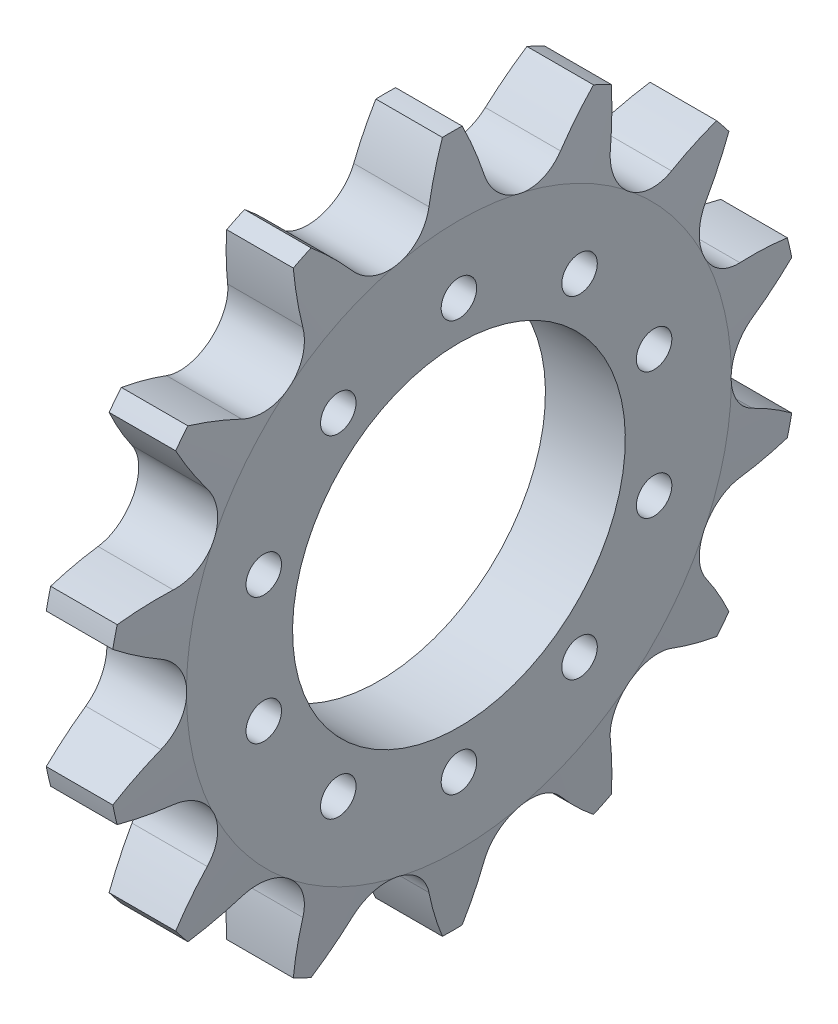
SolidWorks part; units mm, degrees
material "铸造合金钢"
ref_plane "Front Plane" through (0, 0, 0) normal (0, 0, 1) x (1, 0, 0)
ref_plane "Top Plane" through (0, 0, 0) normal (0, 1, 0) x (1, 0, 0)
ref_plane "Right Plane" through (0, 0, 0) normal (1, 0, 0) x (0, 0, -1)
sketch "Sketch1" plane through (0, 0, 0) normal (0, 0, 1) x (1, 0, 0)
  line L0 (15, 156) -> (-15, 156)
  line L1 (0, -55) -> (0, 55) construction
  line L2 (-15, 156) -> (-18, 122.845)
  line L3 (-18, 122.845) -> (-18, 75)
  line L4 (-18, 75) -> (18, 75)
  line L5 (0, 55.746) -> (0, 0) construction
  line L6 (0, 0) -> (-42.4498, 0) construction
  line L7 (18, 122.845) -> (18, 75)
  line L8 (15, 156) -> (18, 122.845)
  line L9 (15, -156) -> (18, -122.845) construction
  line L10 (18, -122.845) -> (18, -75) construction
  line L11 (-18, -75) -> (18, -75) construction
  line L12 (-18, -122.845) -> (-18, -75) construction
  line L13 (-15, -156) -> (-18, -122.845) construction
  line L14 (15, -156) -> (-15, -156) construction
  point P12 (0, 75)
  point P14 (0, 156)
  point P20 (0, -156)
  point P21 (0, -75)
  dimension "D1" = 30
  dimension "D2" = 36
  dimension "D3" = 312
  dimension "D4" = 245.69
  dimension "D5" = 150
revolve "Revolve1" add sketch "Sketch1" angle 360 about L6
sketch "Sketch3" plane through (0, 0, 0) normal (1, 0, 0) x (0, 0, -1)
  line L1 (-159.75, 0) -> (159.75, 0) construction
  line L2 (0, 159.75) -> (0, -159.75) construction
  circle A0 centre (0, 0) radius 196.1047
  arc A3 (153.6801, 30.8707) -> (151.8553, 38.8657) centre (0, 0) ccw
  arc A4 (125.0666, 94.4928) -> (119.9537, 100.9043) centre (0, 0) ccw
  arc A5 (71.6822, 139.3995) -> (64.2938, 142.9576) centre (0, 0) ccw
  arc A6 (4.1003, 156.6964) -> (-4.1003, 156.6964) centre (0, 0) ccw
  arc A7 (-64.2938, 142.9576) -> (-71.6822, 139.3995) centre (0, 0) ccw
  arc A8 (-119.9537, 100.9043) -> (-125.0666, 94.4928) centre (0, 0) ccw
  arc A9 (-151.8553, 38.8657) -> (-153.6801, 30.8707) centre (0, 0) ccw
  arc A10 (-153.6801, -30.8707) -> (-151.8553, -38.8657) centre (0, 0) ccw
  arc A11 (-125.0666, -94.4928) -> (-119.9537, -100.9043) centre (0, 0) ccw
  arc A12 (-71.6822, -139.3995) -> (-64.2938, -142.9576) centre (0, 0) ccw
  arc A13 (-4.1003, -156.6964) -> (4.1003, -156.6964) centre (0, 0) ccw
  arc A14 (64.2938, -142.9576) -> (71.6822, -139.3995) centre (0, 0) ccw
  arc A15 (119.9537, -100.9043) -> (125.0666, -94.4928) centre (0, 0) ccw
  arc A16 (151.8553, -38.8657) -> (153.6801, -30.8707) centre (0, 0) ccw
  arc A17 (153.6801, -30.8707) -> (133.2631, -17.6303) centre (65.3353, -144.7381) ccw
  arc A18 (133.2631, 17.6303) -> (133.2631, -17.6303) centre (142.685, 0) ccw
  arc A19 (133.2631, 17.6303) -> (153.6801, 30.8707) centre (65.3353, 144.7381) ccw
  arc A20 (151.8553, 38.8657) -> (127.7155, 41.9363) centre (121.6646, -102.0566) ccw
  arc A21 (112.4164, 73.7051) -> (127.7155, 41.9363) centre (128.5547, 61.9087) ccw
  arc A22 (112.4164, 73.7051) -> (125.0666, 94.4928) centre (-3.9344, 158.7524) ccw
  arc A23 (119.9537, 100.9043) -> (96.8722, 93.197) centre (153.8967, -39.1615) ccw
  arc A24 (69.3043, 115.1817) -> (96.8722, 93.197) centre (88.9626, 111.5556) ccw
  arc A25 (69.3043, 115.1817) -> (71.6822, 139.3995) centre (-72.4249, 141.3239) ccw
  arc A26 (64.2938, 142.9576) -> (46.8421, 125.9988) centre (155.6477, 31.49) ccw
  arc A27 (12.4655, 133.8451) -> (46.8421, 125.9988) centre (31.7504, 139.1076) ccw
  arc A28 (12.4655, 133.8451) -> (4.1003, 156.6964) centre (-126.5707, 95.9045) ccw
  arc A29 (-4.1003, 156.6964) -> (-12.4655, 133.8451) centre (126.5707, 95.9045) ccw
  arc A30 (-46.8421, 125.9988) -> (-12.4655, 133.8451) centre (-31.7504, 139.1076) ccw
  arc A31 (-46.8421, 125.9988) -> (-64.2938, 142.9576) centre (-155.6477, 31.49) ccw
  arc A32 (-71.6822, 139.3995) -> (-69.3043, 115.1817) centre (72.4249, 141.3239) ccw
  arc A33 (-96.8722, 93.197) -> (-69.3043, 115.1817) centre (-88.9626, 111.5556) ccw
  arc A34 (-96.8722, 93.197) -> (-119.9537, 100.9043) centre (-153.8967, -39.1615) ccw
  arc A35 (-125.0666, 94.4928) -> (-112.4164, 73.7051) centre (3.9344, 158.7524) ccw
  arc A36 (-127.7155, 41.9363) -> (-112.4164, 73.7051) centre (-128.5547, 61.9087) ccw
  arc A37 (-127.7155, 41.9363) -> (-151.8553, 38.8657) centre (-121.6646, -102.0566) ccw
  arc A38 (-153.6801, 30.8707) -> (-133.2631, 17.6303) centre (-65.3353, 144.7381) ccw
  arc A39 (-133.2631, -17.6303) -> (-133.2631, 17.6303) centre (-142.685, 0) ccw
  arc A40 (-133.2631, -17.6303) -> (-153.6801, -30.8707) centre (-65.3353, -144.7381) ccw
  arc A41 (-151.8553, -38.8657) -> (-127.7155, -41.9363) centre (-121.6646, 102.0566) ccw
  arc A42 (-112.4164, -73.7051) -> (-127.7155, -41.9363) centre (-128.5547, -61.9087) ccw
  arc A43 (-112.4164, -73.7051) -> (-125.0666, -94.4928) centre (3.9344, -158.7524) ccw
  arc A44 (-119.9537, -100.9043) -> (-96.8722, -93.197) centre (-153.8967, 39.1615) ccw
  arc A45 (-69.3043, -115.1817) -> (-96.8722, -93.197) centre (-88.9626, -111.5556) ccw
  arc A46 (-69.3043, -115.1817) -> (-71.6822, -139.3995) centre (72.4249, -141.3239) ccw
  arc A47 (-64.2938, -142.9576) -> (-46.8421, -125.9988) centre (-155.6477, -31.49) ccw
  arc A48 (-12.4655, -133.8451) -> (-46.8421, -125.9988) centre (-31.7504, -139.1076) ccw
  arc A49 (-12.4655, -133.8451) -> (-4.1003, -156.6964) centre (126.5707, -95.9045) ccw
  arc A50 (4.1003, -156.6964) -> (12.4655, -133.8451) centre (-126.5707, -95.9045) ccw
  arc A51 (46.8421, -125.9988) -> (12.4655, -133.8451) centre (31.7504, -139.1076) ccw
  arc A52 (46.8421, -125.9988) -> (64.2938, -142.9576) centre (155.6477, -31.49) ccw
  arc A53 (71.6822, -139.3995) -> (69.3043, -115.1817) centre (-72.4249, -141.3239) ccw
  arc A54 (96.8722, -93.197) -> (69.3043, -115.1817) centre (88.9626, -111.5556) ccw
  arc A55 (96.8722, -93.197) -> (119.9537, -100.9043) centre (153.8967, 39.1615) ccw
  arc A56 (125.0666, -94.4928) -> (112.4164, -73.7051) centre (-3.9344, -158.7524) ccw
  arc A57 (127.7155, -41.9363) -> (112.4164, -73.7051) centre (128.5547, -61.9087) ccw
  arc A58 (127.7155, -41.9363) -> (151.8553, -38.8657) centre (121.6646, 102.0566) ccw
extrude "Cut-Extrude1" cut sketch "Sketch3" against normal through all and the other way through all
sketch "Sketch4" plane through (0, 0, 0) normal (1, 0, 0) x (0, 0, -1)
  line L0 (0, 19.8) -> (0, -19.8) construction
  circle A0 centre (0, 92.5) radius 8
  circle A1 centre (0, 0) radius 92.5 construction
  dimension "D1" = 16
  dimension "D2" = 185
extrude "Cut-Extrude2" cut sketch "Sketch4" against normal through all and the other way through all
pattern_circular "CirPattern1" count 10 over 360 about axis through (0, 0, 0) along (1, 0, 0) of "Cut-Extrude2"
